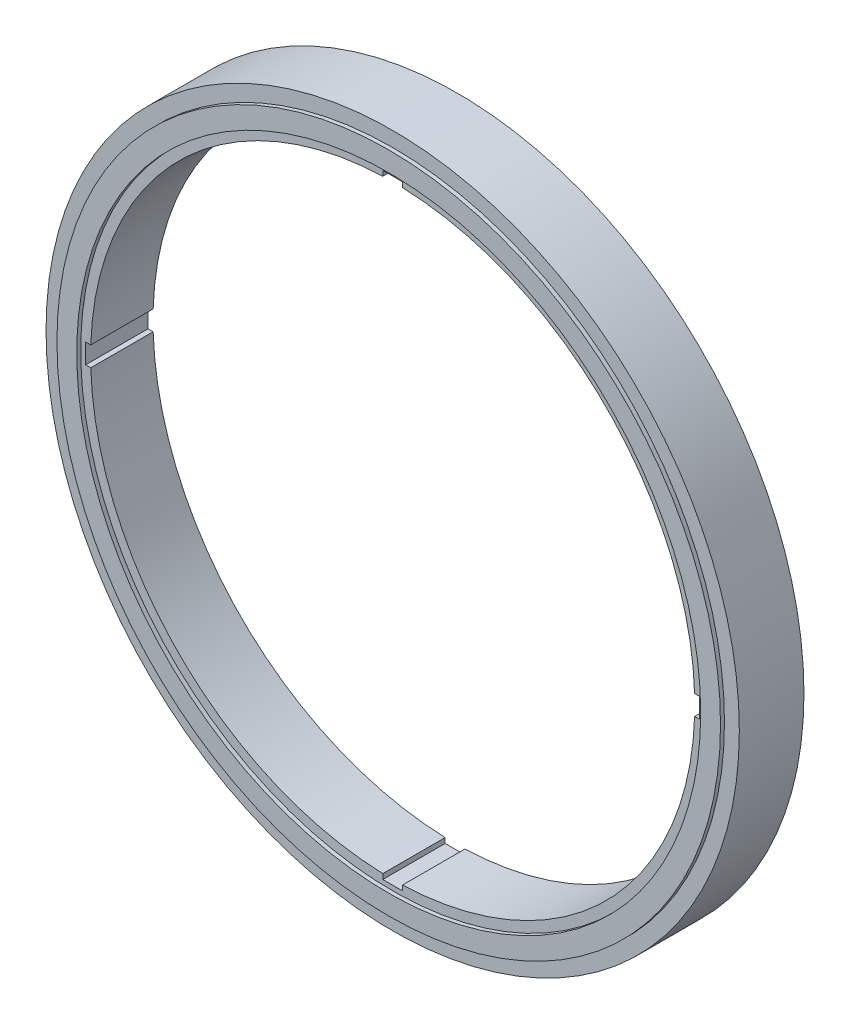
SolidWorks part; units mm, degrees
ref_plane "Front Plane" through (0, 0, 0) normal (0, 0, 1) x (1, 0, 0)
ref_plane "Top Plane" through (0, 0, 0) normal (0, 1, 0) x (1, 0, 0)
ref_plane "Right Plane" through (0, 0, 0) normal (1, 0, 0) x (0, 0, -1)
sketch "Sketch1" plane through (0, 0, 0) normal (0, 0, 1) x (1, 0, 0)
  circle A0 centre (0, 0) radius 175
  dimension "D1" = 350
extrude "Boss-Extrude1" add sketch "Sketch1" along normal blind 35
cosmetic thread "Cosmetic Thread1" parameters "D2"=160.872
sketch "Sketch2" plane through (0, 0, 35) normal (0, 0, 1) x (1, 0, 0)
  circle A0 centre (0, 0) radius 157.5 construction
  circle A1 centre (0, 0) radius 167.5
  circle A3 centre (0, 0) radius 175
  circle A4 centre (0, 0) radius 175
  dimension "D1" = 315
  dimension "D2" = 10
  dimension "D3" = 0
extrude "Cut-Extrude1" cut sketch "Sketch2" against normal blind 2
sketch "Sketch3" plane through (0, 0, 35) normal (0, 0, 1) x (1, 0, 0)
  circle A0 centre (0, 0) radius 157.5
  dimension "D1" = 315
extrude "Cut-Extrude2" cut sketch "Sketch3" against normal blind 2
sketch "Sketch4" plane through (0, 0, 0) normal (0, 0, -1) x (-1, 0, 0)
  circle A0 centre (0, 0) radius 165
  dimension "D1" = 330
extrude "Cut-Extrude3" cut sketch "Sketch4" against normal blind 1.5
sketch "Sketch5" plane through (0, 0, 1.5) normal (0, 0, -1) x (-1, 0, 0)
  circle A0 centre (0, 0) radius 152.5
  dimension "D1" = 305
extrude "Cut-Extrude4" cut sketch "Sketch5" against normal through all
sketch "Sketch7" plane through (0, 0, 1.5) normal (0, 0, -1) x (-1, 0, 0)
  line L1 (-5, -155) -> (5, -155)
  line L2 (-5, -155) -> (-5, 155)
  line L3 (-5, 155) -> (5, 155)
  line L4 (5, -155) -> (5, 155)
  line L5 (-5, -155) -> (5, 155) construction
  line L6 (-5, 155) -> (5, -155) construction
  point P0 (0, 0)
  dimension "D1" = 310
  dimension "D2" = 10
extrude "Cut-Extrude6" cut sketch "Sketch7" against normal blind 99.5
pattern_circular "CirPattern1" count 4 over 360 about axis through (0, 0, 0) along (0, 0, 1) of "Cut-Extrude6"
sketch "Sketch8" plane through (0, 0, 0) normal (0, 0, -1) x (-1, 0, 0)
  circle A0 centre (0, 0) radius 172
  circle A1 centre (0, 0) radius 165 construction
  dimension "D1" = 7
extrude "Cut-Extrude7" cut sketch "Sketch8" against normal blind 99.5 draft 83 flip side to cut
